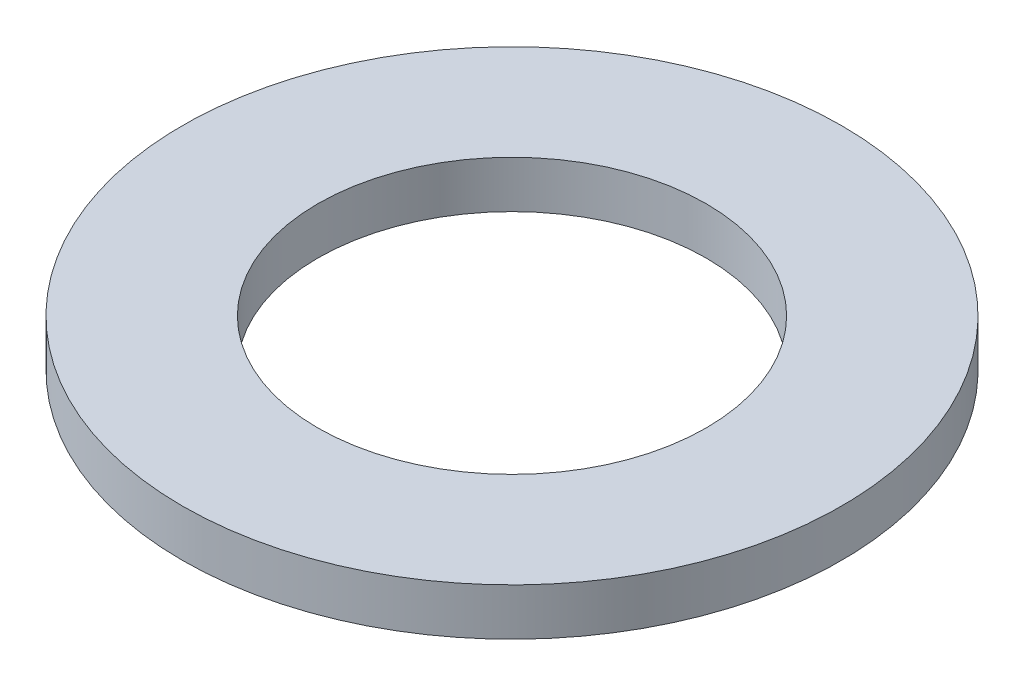
SolidWorks part; units mm, degrees
material "Q235"
ref_plane "Plane1" through (0, 0, 0) normal (0, 0, 1) x (1, 0, 0)
ref_plane "Plane2" through (0, 0, 0) normal (0, 1, 0) x (1, 0, 0)
ref_plane "Plane3" through (0, 0, 0) normal (1, 0, 0) x (0, 0, -1)
sketch "Dimension sketch" plane through (0, 0, 0) normal (0, 0, 1) x (1, 0, 0)
  line L0 (0, 0) -> (56, 0) construction
  point P3 (4, 0)
  point P4 (56, 0)
  point P5 (33, 0)
  dimension "h" = 4
  dimension "d2" = 56
  dimension "d1" = 33
sketch "Sketch1" plane through (0, 0, 0) normal (0, 0, 1) x (1, 0, 0)
  line L0 (0, 0) -> (0, 52.7318) construction
  line L2 (-16.5, 8.6445) -> (-28, 8.6445)
  line L3 (-16.5, 8.6445) -> (-16.5, 12.6445)
  line L4 (-16.5, 12.6445) -> (-28, 12.6445)
  line L5 (-28, 8.6445) -> (-28, 12.6445)
  dimension "D1" = 16.5
  dimension "D2" = 28
  dimension "h" = 4
revolve "Base-Revolve" add sketch "Sketch1" angle 360 about L0
